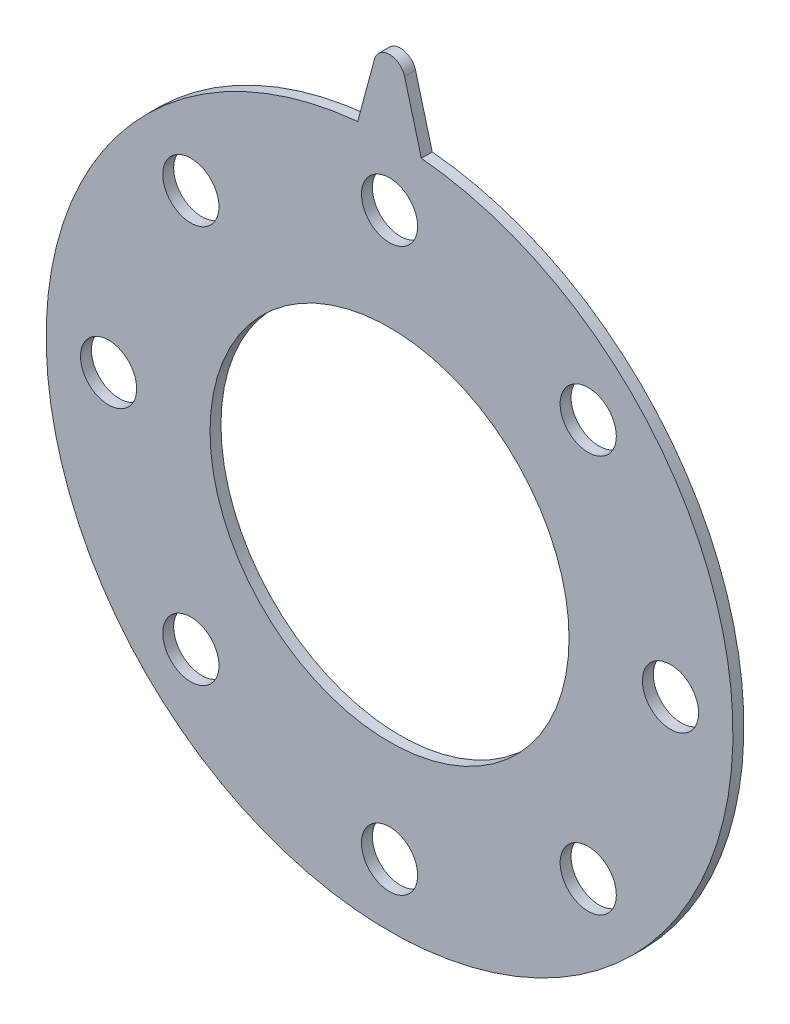
from build123d import *

# Parameters (mm, degrees)
SKETCH1_R           = 57.5
SKETCH1_R_2         = 9
BOSS_EXTRUDE1_DEPTH = 3.5


with BuildPart() as part:
    # Sketch1 → Boss-Extrude1 (new body)
    with BuildSketch(Plane.XY):
        with BuildLine():
            Line((-4.829629131, 129.527129815), (-10.18861298, 109.527129815))
            ThreePointArc((-10.18861298, 109.527129815), (0, -110), (10.18861298, 109.527129815))
            Line((10.18861298, 109.527129815), (4.829629131, 129.527129815))
            ThreePointArc((4.829629131, 129.527129815), (0, 133.23303459), (-4.829629131, 129.527129815))
        make_face()
        Circle(SKETCH1_R, mode=Mode.SUBTRACT)
        with Locations((0, 90)):
            Circle(SKETCH1_R_2, mode=Mode.SUBTRACT)
        with Locations((63.639610307, 63.639610307)):
            Circle(SKETCH1_R_2, mode=Mode.SUBTRACT)
        with Locations((90, 0)):
            Circle(SKETCH1_R_2, mode=Mode.SUBTRACT)
        with Locations((63.639610307, -63.639610307)):
            Circle(SKETCH1_R_2, mode=Mode.SUBTRACT)
        with Locations((0, -90)):
            Circle(SKETCH1_R_2, mode=Mode.SUBTRACT)
        with Locations((-63.639610307, -63.639610307)):
            Circle(SKETCH1_R_2, mode=Mode.SUBTRACT)
        with Locations((-90, 0)):
            Circle(SKETCH1_R_2, mode=Mode.SUBTRACT)
        with Locations((-63.639610307, 63.639610307)):
            Circle(SKETCH1_R_2, mode=Mode.SUBTRACT)
    extrude(amount=BOSS_EXTRUDE1_DEPTH)


solid = part.part
